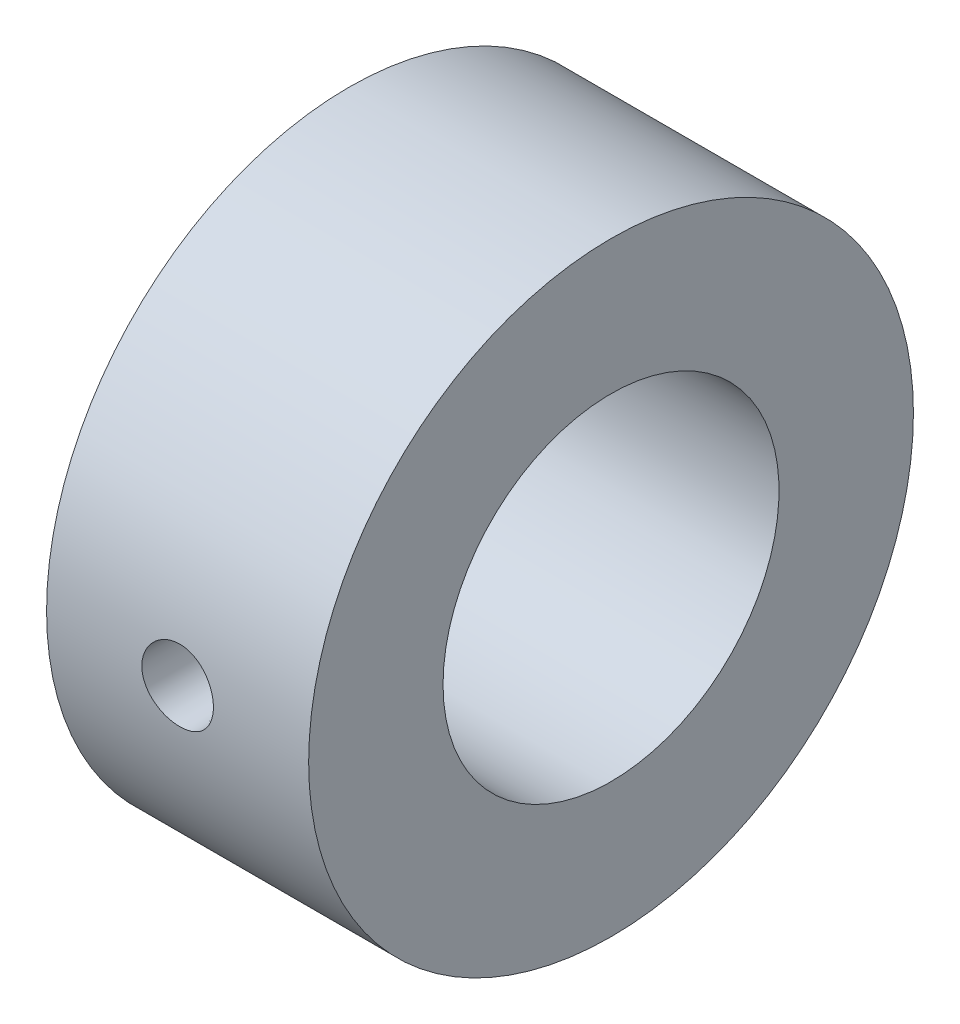
SolidWorks part; units mm, degrees
ref_plane "Front Plane" through (0, 0, 0) normal (0, 0, 1) x (1, 0, 0)
ref_plane "Top Plane" through (0, 0, 0) normal (0, 1, 0) x (1, 0, 0)
ref_plane "Right Plane" through (0, 0, 0) normal (1, 0, 0) x (0, 0, -1)
other "Configuration Table"
ref_plane "Plane1" through (128, 0, 0) normal (-1, 0, 0) x (0, 0, 1)
sketch "Sketch1" plane through (128, 0, 0) normal (-1, 0, 0) x (0, 0, 1)
  circle A0 centre (-102.5, 90) radius 25
  circle A1 centre (-102.5, 90) radius 45
  dimension "D1" = 50
  dimension "D2" = 90
extrude "Boss-Extrude1" add sketch "Sketch1" against normal blind 39
sketch "Sketch2" plane through (147.5, 0, 0) normal (1, 0, 0) x (0, 0, -1)
  line L0 (102.5, 90) -> (-26.3532, 90) construction
  line L4 (0, 90) -> (0, 95.9)
  line L13 (0, 95.9) -> (90, 95)
  line L14 (90, 95) -> (90, 90)
  line L15 (90, 90) -> (0, 90)
  line L16 (0, 30) -> (0, 150) construction
  dimension "D2" = 5.9
  dimension "D1" = 5
  dimension "D3" = 90
revolve "Cut-Revolve1" cut sketch "Sketch2" angle 360 about L0
